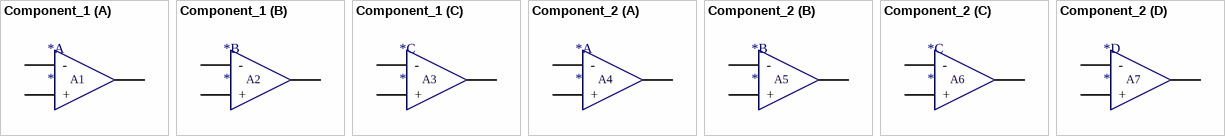
[diagram p0: symbols Component_1 to Component_2]
# Altium schematic symbol library MISC82823-4.SchLib: 2 symbols
Pins are listed as number, name and electrical type; pins without a type are passive.


## Component_1
designator *
part A pins: 2 -, 3 +, 4 +
part B pins: 5 -, 6 +, 7 +
part C pins: 8 -, 9 +, 10 +

## Component_2
designator *
part A pins: 2 -, 3 +, 4 +
part B pins: 5 -, 6 +, 7
part C pins: 8 -, 9 +, 10 +
part D pins: 11 -, 12 +, 13 +